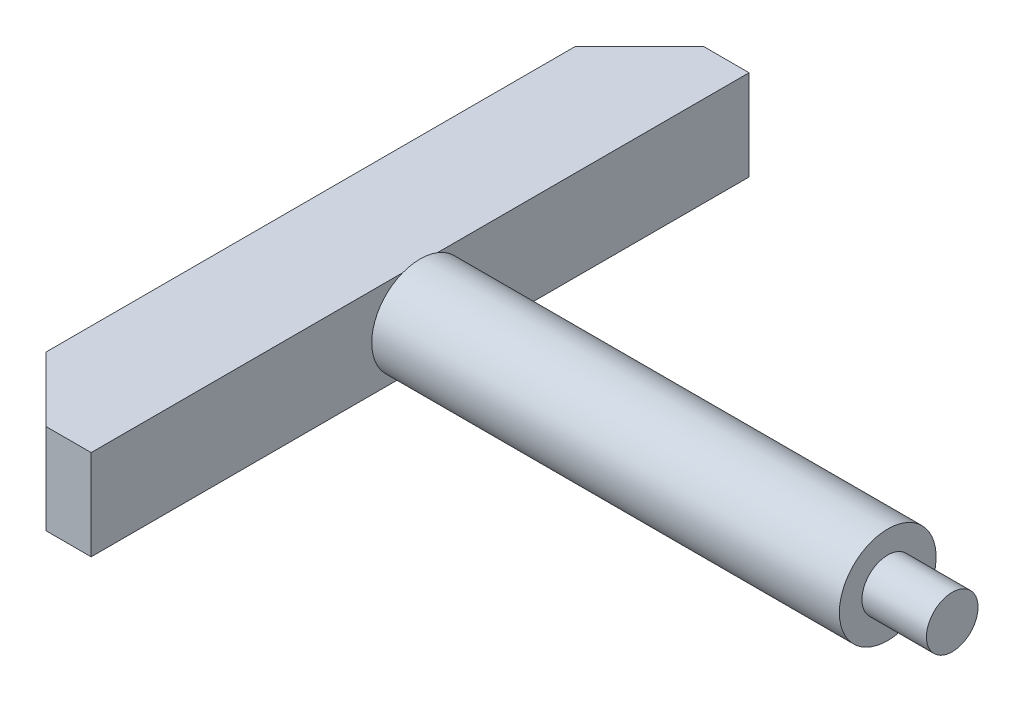
SolidWorks part; units mm, degrees
material "Q235A"
ref_plane "Front Plane" through (0, 0, 0) normal (0, 0, 1) x (1, 0, 0)
ref_plane "Top Plane" through (0, 0, 0) normal (0, 1, 0) x (1, 0, 0)
ref_plane "Right Plane" through (0, 0, 0) normal (1, 0, 0) x (0, 0, -1)
sketch "Sketch1" plane through (0, 0, 0) normal (0, 0, 1) x (1, 0, 0)
  line L0 (0, 0) -> (206.8, 0) construction
  line L1 (0, 0) -> (0, 15)
  line L2 (0, 15) -> (145, 15)
  line L3 (145, 15) -> (145, 8)
  line L4 (145, 8) -> (165, 8)
  line L5 (165, 8) -> (165, 0)
  line L6 (0, 0) -> (165, 0)
  dimension "D1" = 16
  dimension "D2" = 30
  dimension "D3" = 20
  dimension "D4" = 145
revolve "Revolve1" add sketch "Sketch1" angle 360 about L0
sketch "Sketch2" plane through (0, 0, 0) normal (-1, 0, 0) x (0, 0, 1)
  line L1 (102, -14) -> (-102, -14)
  line L2 (102, -14) -> (102, 14)
  line L3 (102, 14) -> (-102, 14)
  line L4 (-102, -14) -> (-102, 14)
  line L5 (102, -14) -> (-102, 14) construction
  line L6 (102, 14) -> (-102, -14) construction
  point P0 (0, 0)
  dimension "D1" = 204
  dimension "D2" = 28
extrude "Boss-Extrude1" add sketch "Sketch2" along normal blind 34
chamfer "Chamfer1" distance 20 angle 45 2 edges at (-34, 0, 102) (-34, 0, -102)
